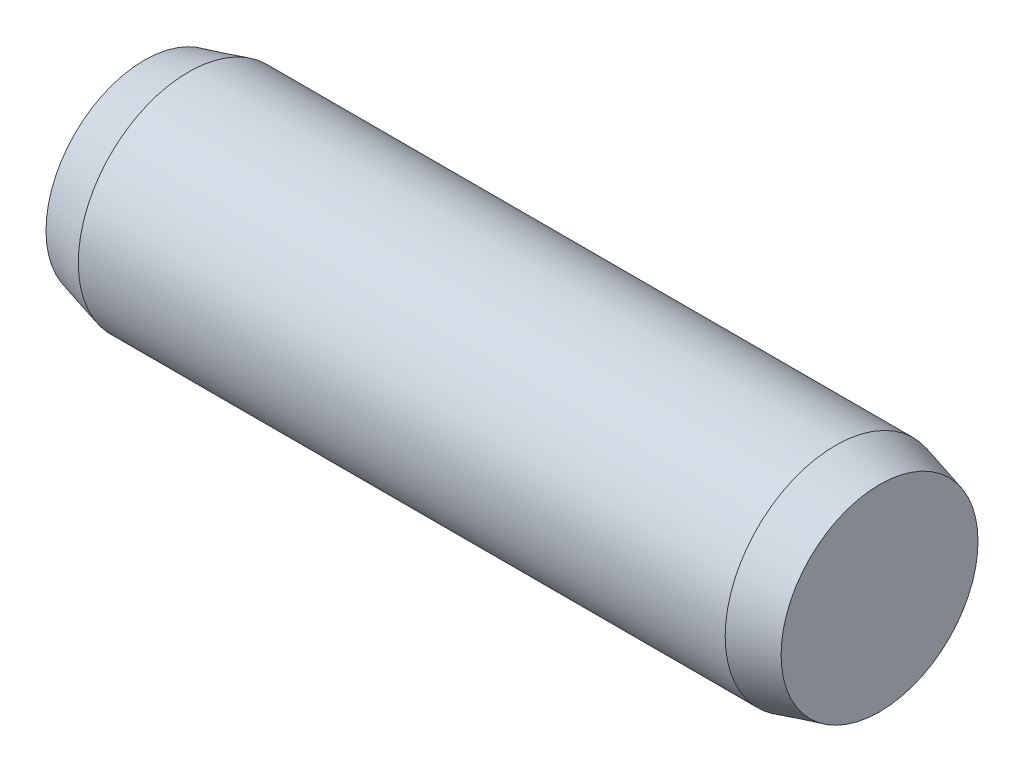
SolidWorks part; units mm, degrees
ref_plane "Front" through (0, 0, 0) normal (0, 0, 1) x (1, 0, 0)
ref_plane "Top" through (0, 0, 0) normal (0, 1, 0) x (1, 0, 0)
ref_plane "Right" through (0, 0, 0) normal (1, 0, 0) x (0, 0, -1)
other "Configuration Table"
sketch "Sketch1" plane through (0, 0, 0) normal (0, 0, 1) x (1, 0, 0)
  line L0 (0, 0) -> (2, 0)
  line L1 (2, 0) -> (2, 0.2678)
  line L2 (2, 0.2678) -> (1.88, 0.3)
  line L3 (1.88, 0.3) -> (0.12, 0.3)
  line L4 (0.12, 0.3) -> (0, 0.2678)
  line L5 (0, 0.2678) -> (0, 0)
  line L6 (-1.6557, 0) -> (2.6973, 0) construction
revolve "Base-Revolve" add sketch "Sketch1" angle 360 about L6
equation "\"D6@Sketch1\" = \"c@Sketch1\""
